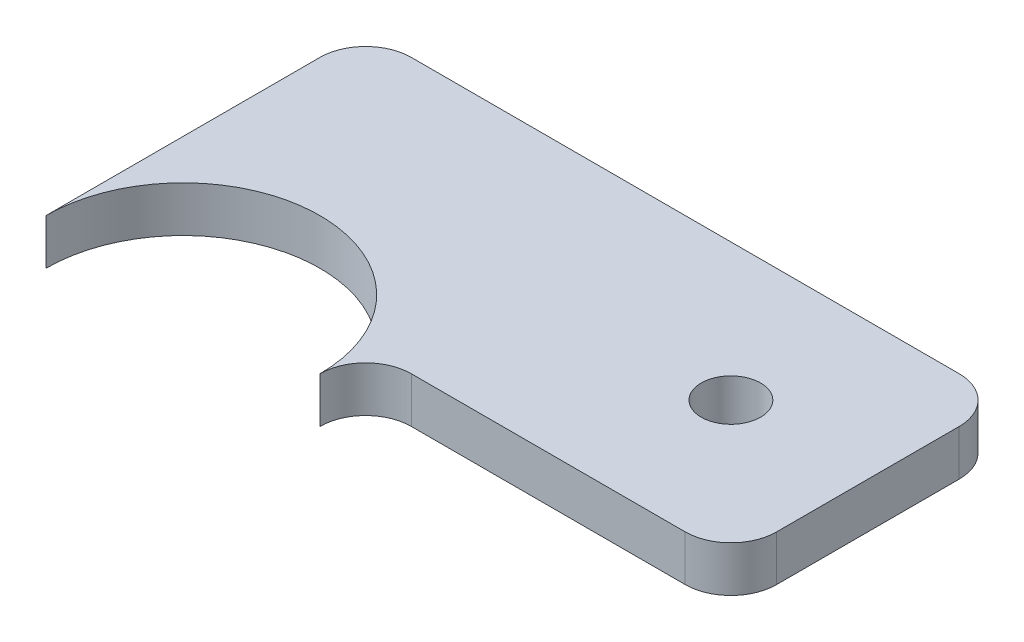
SolidWorks part; units mm, degrees
material "1023 碳钢板 (SS)"
ref_plane "Front Plane" through (0, 0, 0) normal (0, 0, 1) x (1, 0, 0)
ref_plane "Top Plane" through (0, 0, 0) normal (0, 1, 0) x (1, 0, 0)
ref_plane "Right Plane" through (0, 0, 0) normal (1, 0, 0) x (0, 0, -1)
sketch "Sketch1" plane through (0, 210, 0) normal (0, 1, 0) x (1, 0, 0)
  line L2 (-15, 0) -> (-15, 35)
  line L3 (-15, 35) -> (55, 35)
  line L4 (55, 5) -> (55, 35)
  line L5 (14.1421, 5) -> (55, 5)
  circle A0 centre (0, 0) radius 15 construction
  arc A1 (14.1421, 5) -> (-15, 0) centre (0, 0) ccw
  point P3 (55, 0)
extrude "Boss-Extrude1" add sketch "Sketch1" against normal blind 5
fillet "Fillet1" radius 5 3 edges at (55, 207.5, -35) (-15, 207.5, -35) (55, 207.5, -5)
sketch "Sketch2" plane through (0, 210, 0) normal (0, 1, 0) x (1, 0, 0)
  line L0 (55, 10) -> (55, 30) construction
  line L1 (50, 35) -> (-10, 35) construction
  circle A0 centre (40, 20) radius 3.25
  dimension "D1" = 15
  dimension "D2" = 15
extrude "Cut-Extrude1" cut sketch "Sketch2" against normal blind 5
sketch "Sketch3" plane through (0, 210, 0) normal (0, 1, 0) x (1, 0, 0)
  line L0 (14.1421, 5) -> (50, 5) construction
  line L1 (20, 5) -> (50, 5)
  line L2 (20, 5) -> (14.1421, 5)
  arc A2 (15, 0) -> (20, 5) centre (20, 0) cw
  circle A3 centre (0, 0) radius 15 construction
  arc A4 (15, 0) -> (14.1421, 5) centre (0, 0) ccw
  line M9 (14.1421, 5) -> (50, 5)
  dimension "D1" = 5
extrude "Boss-Extrude2" add sketch "Sketch3" against normal blind 5 contours A4 A2 M9
